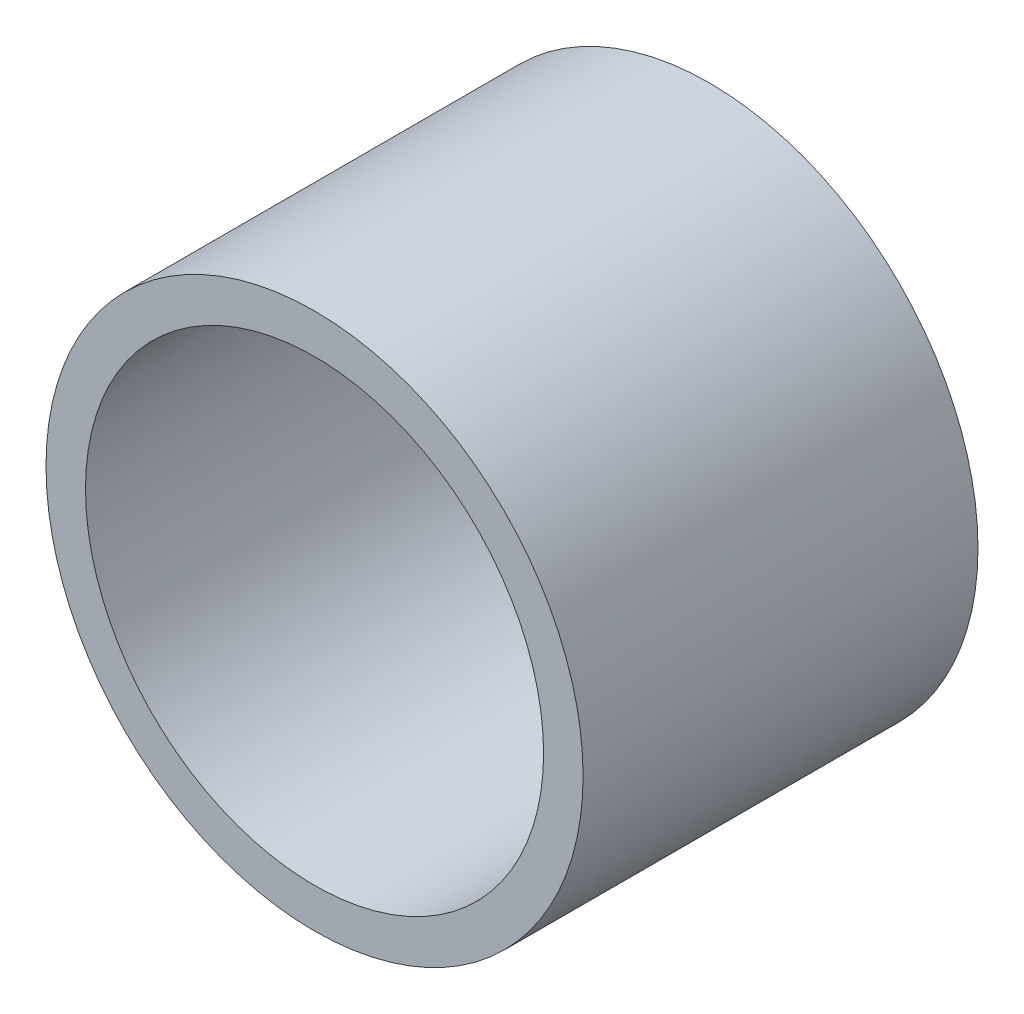
SolidWorks part; units mm, degrees
ref_plane "Front Plane" through (0, 0, 0) normal (0, 0, 1) x (1, 0, 0)
ref_plane "Top Plane" through (0, 0, 0) normal (0, 1, 0) x (1, 0, 0)
ref_plane "Right Plane" through (0, 0, 0) normal (1, 0, 0) x (0, 0, -1)
sketch "Sketch1" plane through (0, 0, 0) normal (0, 0, 1) x (1, 0, 0)
  circle A1 centre (0, 0) radius 34
extrude "Boss-Extrude1" add sketch "Sketch1" along normal blind 50
shell "Shell1" thickness 5
